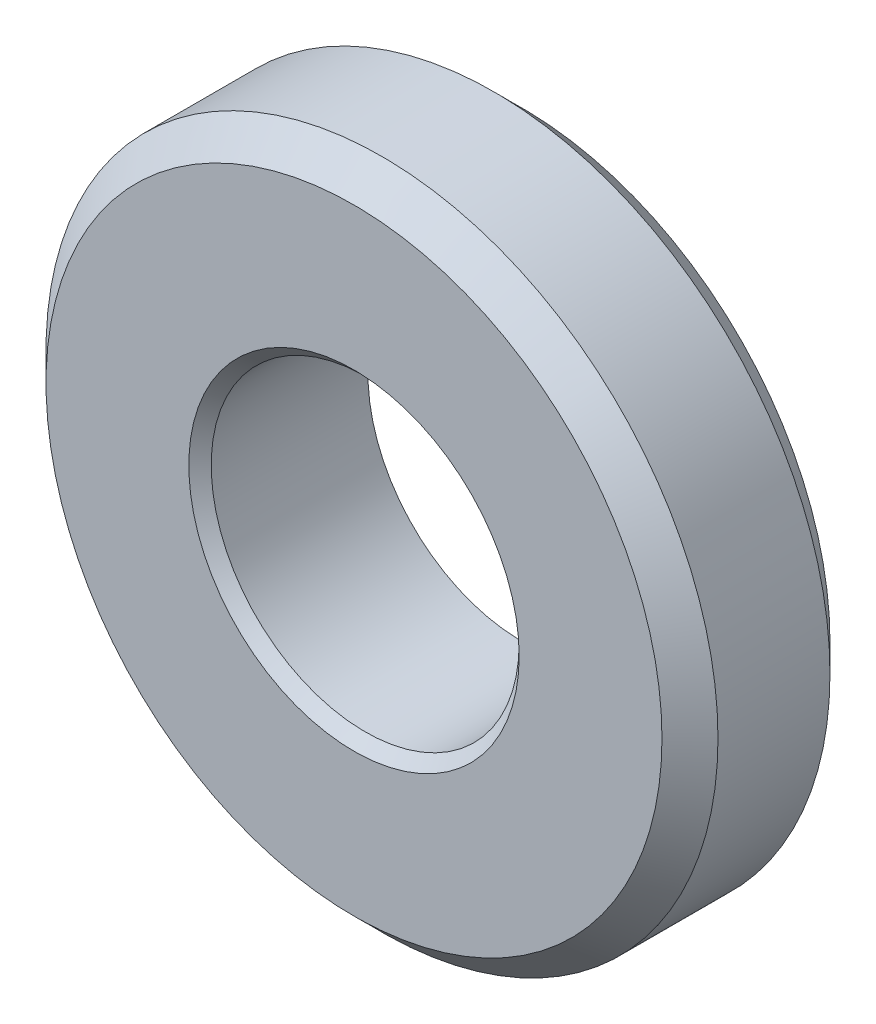
from build123d import *

# Parameters (mm, degrees)
SKETCH1_R           = 60
SKETCH1_R_2         = 27.5
BOSS_EXTRUDE1_DEPTH = 30
CHAMFER1_SIZE       = 5
CHAMFER2_SIZE       = 2


with BuildPart() as part:
    # Sketch1 → Boss-Extrude1 (new body)
    with BuildSketch(Plane.XY):
        Circle(SKETCH1_R)
        Circle(SKETCH1_R_2, mode=Mode.SUBTRACT)
    extrude(amount=BOSS_EXTRUDE1_DEPTH)

    # Chamfer1
    chamfer1_edges = [part.edges().sort_by_distance(p)[0] for p in [
        (-60, 0, 0),
        (-60, 0, 30),
    ]]
    chamfer(chamfer1_edges, length=CHAMFER1_SIZE)

    # Chamfer2
    chamfer2_edges = [part.edges().sort_by_distance(p)[0] for p in [
        (-27.5, 0, 30),
    ]]
    chamfer(chamfer2_edges, length=CHAMFER2_SIZE)


solid = part.part
